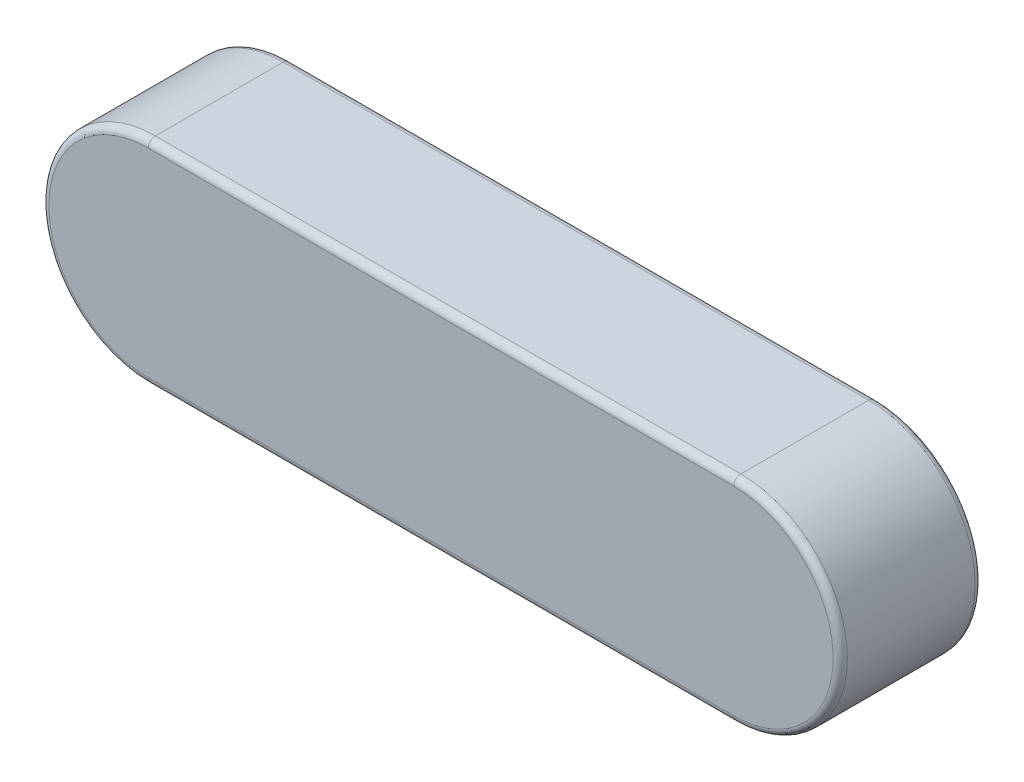
from build123d import *

# Parameters (mm, degrees)
BOSS_EXTRUDE_DEPTH = 8
FILLET1_R          = 0.4


with BuildPart() as part:
    # Sketch1 → Boss-Extrude (new body)
    with BuildSketch(Plane.XY):
        with BuildLine():
            Line((-16.5, 6), (16.5, 6))
            ThreePointArc((16.5, 6), (22.5, 0), (16.5, -6))
            Line((16.5, -6), (-16.5, -6))
            ThreePointArc((-16.5, -6), (-22.5, 0), (-16.5, 6))
        make_face()
    extrude(amount=BOSS_EXTRUDE_DEPTH)

    # Fillet1
    fillet1_edges = [part.edges().sort_by_distance(p)[0] for p in [
        (22.5, 0, 8),
        (0, 6, 8),
        (-22.5, 0, 8),
        (0, 6, 0),
        (22.5, 0, 0),
        (0, -6, 0),
        (-22.5, 0, 0),
        (0, -6, 8),
    ]]
    fillet(fillet1_edges, radius=FILLET1_R)


solid = part.part
